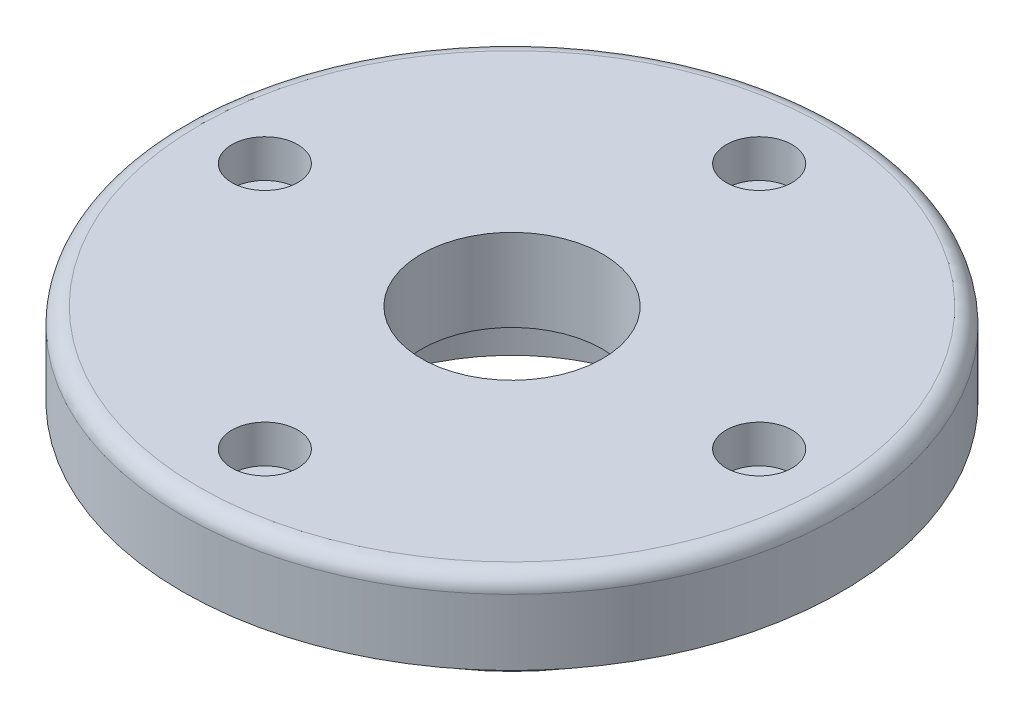
from build123d import *

# Parameters (mm, degrees)
SKETCH1_R                                          = 26
SKETCH1_R_2                                        = 21
BOSS_EXTRUDE1_DEPTH                                = 10
SKETCH2_R                                          = 40
BOSS_EXTRUDE2_DEPTH                                = 10
SKETCH3_R                                          = 11
CUT_EXTRUDE1_DEPTH                                 = 10
FILLET1_R                                          = 2
HOLE_SIZE_BASED_HEX_SOCKET_HEAD_CAP_SC_D           = 4.5
HOLE_SIZE_BASED_HEX_SOCKET_HEAD_CAP_SC_CBORE_D     = 8
HOLE_SIZE_BASED_HEX_SOCKET_HEAD_CAP_SC_CBORE_DEPTH = 4.6
CIRPATTERN1_COUNT                                  = 4


with BuildPart() as part:
    # Sketch1 → Boss-Extrude1 (new body)
    with BuildSketch(Plane(origin=(0, 0, 0), x_dir=(1, 0, 0), z_dir=(0, 1, 0))):
        with Locations(Location((0, 0, 0), (0, 0, 270))):
            Circle(SKETCH1_R)
        with Locations(Location((0, 0, 0), (0, 0, 270))):
            Circle(SKETCH1_R_2, mode=Mode.SUBTRACT)
    extrude(amount=BOSS_EXTRUDE1_DEPTH)

    # Sketch2 → Boss-Extrude2 (add)
    with BuildSketch(Plane(origin=(0, 10, 0), x_dir=(1, 0, 0), z_dir=(0, 1, 0))):
        with Locations(Location((0, 0, 0), (0, 0, 270))):
            Circle(SKETCH2_R)
    extrude(amount=BOSS_EXTRUDE2_DEPTH)

    # Sketch3 → Cut-Extrude1 (cut)
    with BuildSketch(Plane.XZ.offset(-10)):
        with Locations(Location((0, 0, 0), (0, 0, 270))):
            Circle(SKETCH3_R)
    extrude(amount=-CUT_EXTRUDE1_DEPTH, mode=Mode.SUBTRACT)

    # Fillet1
    fillet1_edges = [part.edges().sort_by_distance(p)[0] for p in [
        (0, 20, -40),
    ]]
    fillet(fillet1_edges, radius=FILLET1_R)

    # Hole size (%based) hex socket head cap screw type 1 (through all)
    with Locations(Plane(origin=(0, 20, 0), x_dir=(1, 0, 0), z_dir=(0, 1, 0))):
        with Locations((0, 30)):
            hole_size_based_hex_socket_head_cap_sc = CounterBoreHole(HOLE_SIZE_BASED_HEX_SOCKET_HEAD_CAP_SC_D / 2, HOLE_SIZE_BASED_HEX_SOCKET_HEAD_CAP_SC_CBORE_D / 2, HOLE_SIZE_BASED_HEX_SOCKET_HEAD_CAP_SC_CBORE_DEPTH)

    # CirPattern1: Hole size (%based) hex socket head cap screw type 1 ×4 about axis
    cirpattern1_axis = Axis((0, 0, 0), (0, 1, 0))
    for i in range(1, CIRPATTERN1_COUNT):
        add(hole_size_based_hex_socket_head_cap_sc.rotate(cirpattern1_axis, i * 360 / CIRPATTERN1_COUNT), mode=Mode.SUBTRACT)


solid = part.part
